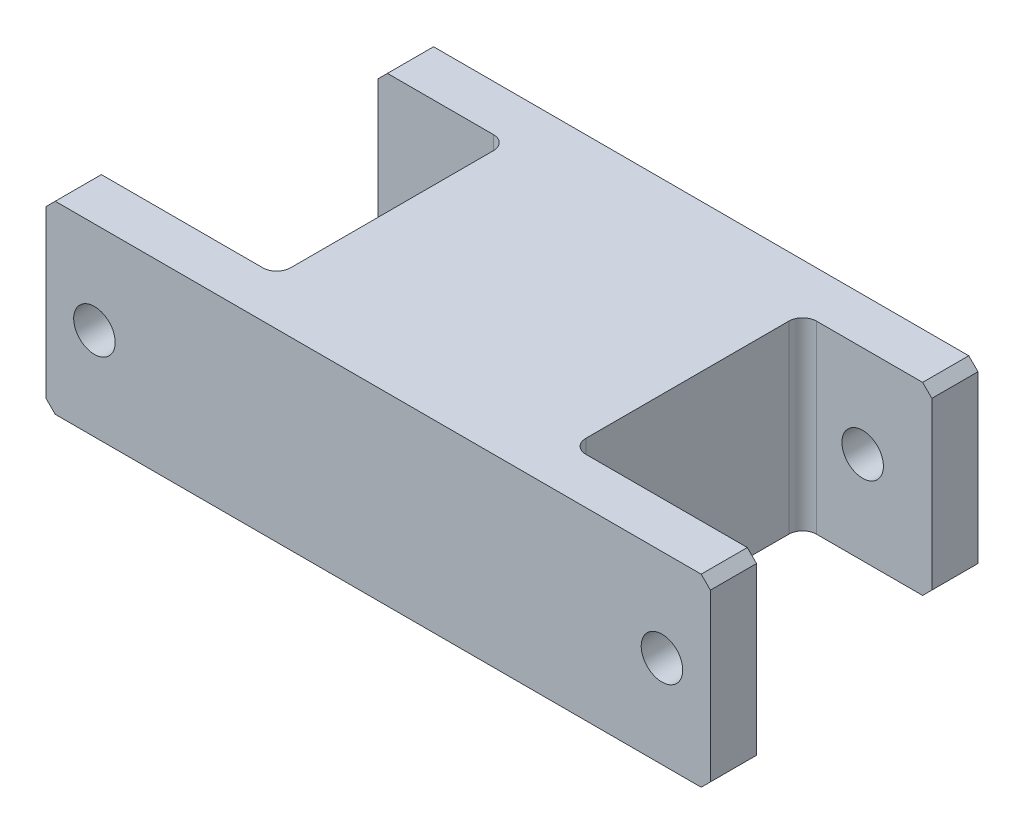
from build123d import *

# Parameters (mm, degrees)
SKETCH_1_W             = 120
SKETCH_1_H             = 40
EXTRUDE_1_DEPTH        = 70
SKETCH_2_R             = 3
CUT_EXTRUDE_1_DEPTH    = 198.553816398
SKETCH_3_W             = 47.323469883
SKETCH_3_H             = 50
CUT_EXTRUDE_2_DEPTH    = 197.577989194
FILLET_1_R             = 3
SKETCH_4_W             = 12
SKETCH_4_H             = 40
EXTRUDE_2_DEPTH        = 10
SKETCH_5_W             = 12
SKETCH_5_H             = 40
EXTRUDE_3_DEPTH        = 10
SKETCH_6_R             = 3
EXTRUDE_4_DEPTH        = 10
SKETCH_7_R             = 4.5
CUT_EXTRUDE_3_DEPTH    = 10
CHAMFER_1_SIZE         = 2
HOLE_WIZARD_M8_1_D     = 9
HOLE_WIZARD_M8_1_DEPTH = 19.75
HOLE_WIZARD_M8_1_TIP   = 2.703872786


with BuildPart() as part:
    # 草图1 → 凸台-拉伸1 (new body)
    with BuildSketch(Plane.XY):
        with Locations((119.284427197, 24.548900527)):
            Rectangle(SKETCH_1_W, SKETCH_1_H)
    extrude(amount=EXTRUDE_1_DEPTH)

    # 草图2 → 切除-拉伸1 (cut, through all)
    with BuildSketch(Plane.XY.offset(70)):
        with Locations((74.284427197, 24.548900527)):
            Circle(SKETCH_2_R)
        with Locations((164.284427197, 24.548900527)):
            Circle(SKETCH_2_R)
    extrude(amount=-CUT_EXTRUDE_1_DEPTH, mode=Mode.SUBTRACT)

    # 草图3 → 切除-拉伸2 (cut, through all)
    with BuildSketch(Plane(origin=(0, 44.548900527, 0), x_dir=(1, 0, 0), z_dir=(0, 1, 0))):
        with Locations((174.946162139, -35)):
            Rectangle(SKETCH_3_W, SKETCH_3_H)
        with Locations((63.622692255, -35)):
            Rectangle(SKETCH_3_W, SKETCH_3_H)
    extrude(amount=-CUT_EXTRUDE_2_DEPTH, mode=Mode.SUBTRACT)

    # 圆角1
    fillet_1_edges = [part.edges().sort_by_distance(p)[0] for p in [
        (151.284427197, 24.548900527, 10),
        (151.284427197, 24.548900527, 60),
        (87.284427197, 24.548900527, 60),
        (87.284427197, 24.548900527, 10),
    ]]
    fillet(fillet_1_edges, radius=FILLET_1_R)

    # 草图4 → 凸台-拉伸2 (add)
    with BuildSketch(Plane(origin=(0, 0, 60), x_dir=(-1, 0, 0), z_dir=(0, 0, -1))):
        with Locations((-185.284427197, 24.548900527)):
            Rectangle(SKETCH_4_W, SKETCH_4_H)
    extrude(amount=-EXTRUDE_2_DEPTH)

    # 草图5 → 凸台-拉伸3 (add)
    with BuildSketch(Plane.XY.offset(70)):
        with Locations((53.284427197, 24.548900527)):
            Rectangle(SKETCH_5_W, SKETCH_5_H)
    extrude(amount=-EXTRUDE_3_DEPTH)

    # 草图6 → 凸台-拉伸4 (add)
    with BuildSketch(Plane.XY.offset(70)):
        with Locations((74.284427197, 24.548900527)):
            Circle(SKETCH_6_R)
        with Locations((164.284427197, 24.548900527)):
            Circle(SKETCH_6_R)
    extrude(amount=-EXTRUDE_4_DEPTH)

    # 草图7 → 切除-拉伸3 (cut)
    with BuildSketch(Plane.XY.offset(70)):
        with Locations((57.784427197, 24.548900527)):
            Circle(SKETCH_7_R)
    cut_extrude_3 = extrude(amount=-CUT_EXTRUDE_3_DEPTH, mode=Mode.SUBTRACT)

    # 镜向2: 切除-拉伸3 across plane
    add(cut_extrude_3.mirror(Plane(origin=(119.284427197, 0, 0), x_dir=(0, 0, 1), z_dir=(1, 0, 0))), mode=Mode.SUBTRACT)

    # 倒角1
    chamfer_1_edges = [part.edges().sort_by_distance(p)[0] for p in [
        (47.284427197, 4.548900527, 65),
        (47.284427197, 44.548900527, 65),
        (179.284427197, 4.548900527, 5),
        (179.284427197, 44.548900527, 5),
        (59.284427197, 4.548900527, 5),
        (59.284427197, 44.548900527, 5),
        (191.284427197, 4.548900527, 65),
        (191.284427197, 44.548900527, 65),
    ]]
    chamfer(chamfer_1_edges, length=CHAMFER_1_SIZE)

    # Hole Wizard M8 _1
    with Locations(Plane(origin=(74.284427197, 24.548900527, 0), x_dir=(-1, 0, 0), z_dir=(0, 0, -1))):
        with Locations((0, 0), (-90, 0)):
            Hole(HOLE_WIZARD_M8_1_D / 2, depth=HOLE_WIZARD_M8_1_DEPTH)
            with Locations((0, 0, -(HOLE_WIZARD_M8_1_DEPTH + HOLE_WIZARD_M8_1_TIP / 2))):  # 118° drill point
                Cone(0, HOLE_WIZARD_M8_1_D / 2, HOLE_WIZARD_M8_1_TIP, mode=Mode.SUBTRACT)


solid = part.part
